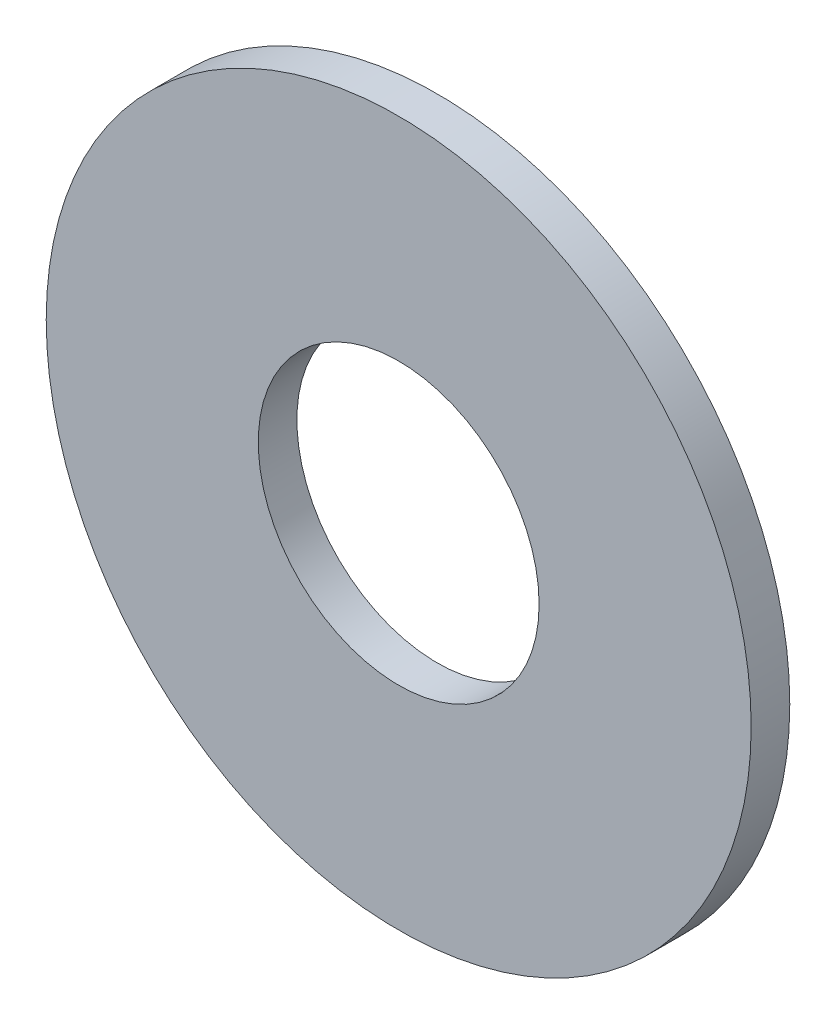
SolidWorks part; units mm, degrees
material "AISI 4130 Steel, normalized at 870C"
ref_plane "Front" through (0, 0, 0) normal (0, 0, 1) x (1, 0, 0)
ref_plane "Top" through (0, 0, 0) normal (0, 1, 0) x (1, 0, 0)
ref_plane "Right" through (0, 0, 0) normal (1, 0, 0) x (0, 0, -1)
sketch "Sketch1" plane through (0, 0, 0) normal (0, 0, 1) x (1, 0, 0)
  circle A0 centre (0, 0) radius 16.002
  circle A1 centre (0, 0) radius 6.3754
  dimension "D1" = 12.7508
  dimension "D2" = 32.004
extrude "Boss-Extrude1" add sketch "Sketch1" along normal blind 1.7526
